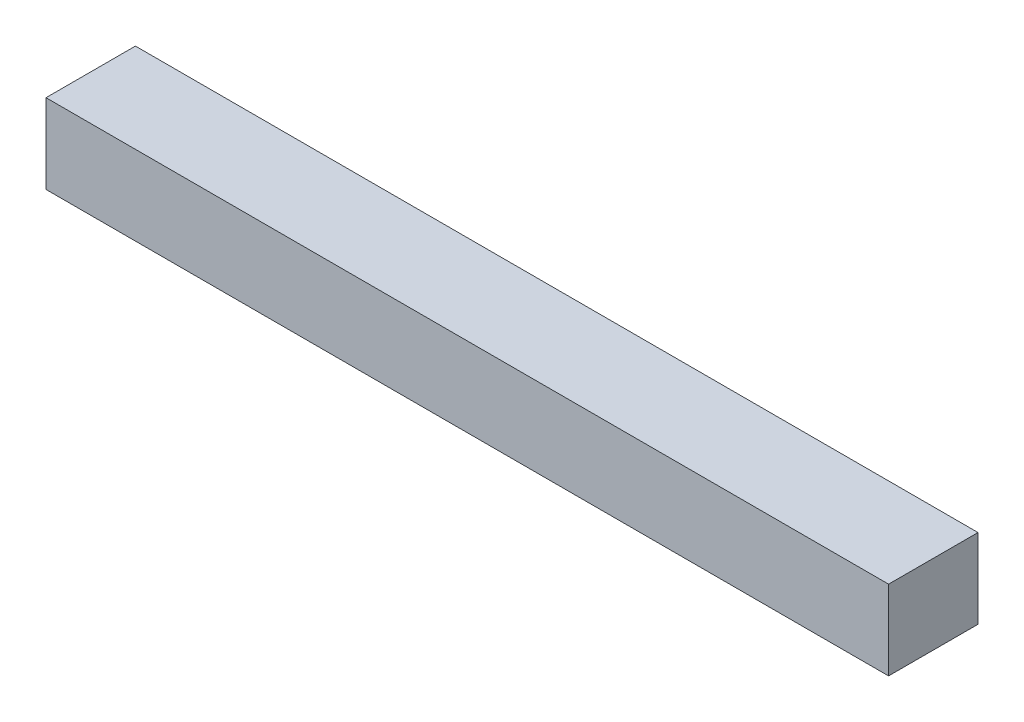
from build123d import *

# Parameters (mm, degrees)
SKETCH_1_W      = 4240
SKETCH_1_H      = 400
EXTRUDE_1_DEPTH = 450


with BuildPart() as part:
    # 草图1 → 凸台-拉伸1 (new body)
    with BuildSketch(Plane.XY):
        Rectangle(SKETCH_1_W, SKETCH_1_H)
    extrude(amount=EXTRUDE_1_DEPTH)


solid = part.part
